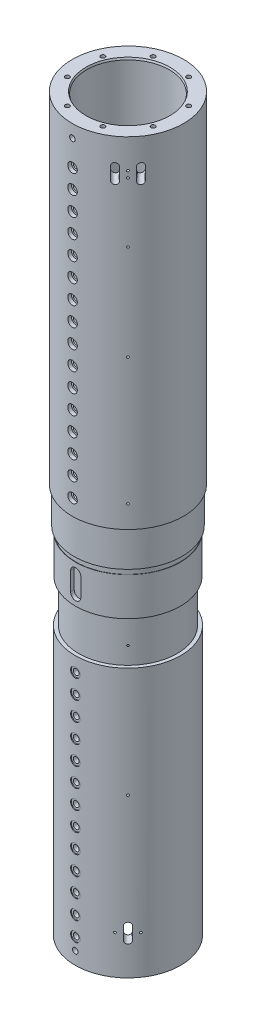
SolidWorks part; units mm, degrees
ref_plane "Front Plane" through (0, 0, 0) normal (0, 0, 1) x (1, 0, 0)
ref_plane "Top Plane" through (0, 0, 0) normal (0, 1, 0) x (1, 0, 0)
ref_plane "Right Plane" through (0, 0, 0) normal (1, 0, 0) x (0, 0, -1)
sketch "Sketch1" plane through (0, 0, 0) normal (0, 1, 0) x (1, 0, 0)
  circle A0 centre (0, 0) radius 65
  circle A1 centre (0, 0) radius 87.5
  dimension "D1" = 130
  dimension "D2" = 175
extrude "Boss-Extrude1" add sketch "Sketch1" along normal blind 1149
hole_wizard "M8 Tapped Hole1" positions "Sketch18" profile "Sketch19" tap size "M8" standard "GB"
sketch "Sketch18" plane through (0, 1149, 0) normal (0, 1, 0) x (1, 0, 0)
  line L0 (0, 0) -> (0, -111.092) construction
  line L2 (27.9359, -67.4432) -> (0, 0) construction
  circle A1 centre (0, 0) radius 73
  point P63 (27.9359, -67.4432)
  dimension "D1" = 146
  dimension "D2" = 22.5
sketch "Sketch19" plane through (27.9359, 1149, 67.4432) normal (1, 0, 0) x (0, 0, 1)
  line L0 (0, 0) -> (0, 33.2929)
  line L1 (0, 33.2929) -> (3.4, 31.25)
  line L2 (3.4, 31.25) -> (3.4, 0)
  line L5 (3.4, 0) -> (0, 0)
  line L10 (0, 33.2929) -> (-3.4, 31.25) construction
  line L11 (0, -6.35) -> (0, 107.95) construction
  dimension "螺纹孔钻头直径" = 6.8
  dimension "螺纹孔钻头深度" = 31.25
  dimension "导头角度" = 118
cosmetic thread "Cosmetic thread 5" parameters "D1"=25, "D2"=8
ref_plane "Plane1" through (0, 574.5, 0) normal (0, 1, 0) x (1, 0, 0)
hole_wizard "M8 Tapped Hole2" positions "Sketch20" profile "Sketch21" tap size "M8" standard "GB"
sketch "Sketch20" plane through (0, 0, 0) normal (0, -1, 0) x (-1, 0, 0)
  line L0 (0, 65) -> (0, 0) construction
  line L3 (0, 0) -> (-27.9359, -67.4432) construction
  circle A1 centre (0, 0) radius 65 construction
  point P0 (-27.9359, -67.4432)
  dimension "D1" = 22.5
  dimension "D2" = 73
sketch "Sketch21" plane through (27.9359, 0, 67.4432) normal (1, 0, 0) x (0, 0, -1)
  line L0 (0, 0) -> (0, 38.2929)
  line L1 (0, 38.2929) -> (3.4, 36.25)
  line L2 (3.4, 36.25) -> (3.4, 0)
  line L5 (3.4, 0) -> (0, 0)
  line L10 (0, 38.2929) -> (-3.4, 36.25) construction
  line L11 (0, -6.35) -> (0, 107.95) construction
  dimension "螺纹孔钻头直径" = 6.8
  dimension "螺纹孔钻头深度" = 36.25
  dimension "导头角度" = 118
cosmetic thread "Cosmetic thread 13" parameters "D1"=30, "D2"=8
pattern_circular "CirPattern1" count 8 over 360 about axis through (0, 0, 0) along (0, 1, 0) of "M8 Tapped Hole2"
ref_plane "Plane2" through (0, 0, 87.5) normal (0, 0, 1) x (1, 0, 0)
hole_wizard "Hole size (% based on socket head cap screw type)3" positions "Sketch23" profile "Sketch25" counterbore size "M8" standard "GB"
sketch "Sketch23" plane through (0, 0, 87.5) normal (0, 0, 1) x (1, 0, 0)
  line L0 (0, 1111.2839) -> (0, 0) construction
  line L3 (87.5, 1149) -> (-87.5, 1149) construction
  line L4 (-87.5, 0) -> (87.5, 0) construction
  point P0 (0, 1089)
  dimension "D1" = 60
sketch "Sketch25" plane through (0, 1089, 87.5) normal (1, 0, 0) x (0, -1, 0)
  line L0 (0, 0) -> (0, 82.7039)
  line L1 (0, 82.7039) -> (4.5, 80)
  line L2 (4.5, 80) -> (4.5, 6)
  line L3 (4.5, 6) -> (7.5, 6)
  line L4 (7.5, 6) -> (7.5, 0)
  line L5 (7.5, 0) -> (0, 0)
  line L10 (0, 82.7039) -> (-4.5, 80) construction
  line L11 (0, -6.35) -> (0, 107.95) construction
  dimension "孔直径" = 9
  dimension "孔深度" = 80
  dimension "柱形沉头孔直径" = 15
  dimension "柱形沉头孔深度" = 6
  dimension "导头角度" = 118
ref_plane "Plane3" through (61.8718, 0, 61.8718) normal (0.7071, 0, 0.7071) x (0, -1, 0)
sketch "Sketch29" plane through (61.8718, 0, 61.8718) normal (0.7071, 0, 0.7071) x (0, -1, 0)
  line L0 (-1108, 14.5) -> (-1088, 14.5) construction
  line L1 (-1108, 19.5) -> (-1088, 19.5)
  line L2 (-1108, 9.5) -> (-1088, 9.5)
  line L3 (-1108, -14.5) -> (-1088, -14.5) construction
  line L4 (-1108, -9.5) -> (-1088, -9.5)
  line L5 (-1108, -19.5) -> (-1088, -19.5)
  line L6 (-1149, 0) -> (-965.5167, 0) construction
  line L7 (-1149, 87.5) -> (-1149, -87.5) construction
  arc A0 (-1108, 19.5) -> (-1108, 9.5) centre (-1108, 14.5) ccw
  arc A1 (-1088, 9.5) -> (-1088, 19.5) centre (-1088, 14.5) ccw
  arc A2 (-1108, -9.5) -> (-1108, -19.5) centre (-1108, -14.5) ccw
  arc A3 (-1088, -19.5) -> (-1088, -9.5) centre (-1088, -14.5) ccw
  point P2 (-1098, 14.5)
  point P8 (-1098, -14.5)
  dimension "D1" = 29
  dimension "D2" = 5
  dimension "D3" = 41
  dimension "D4" = 20
extrude "Cut-Extrude13" cut sketch "Sketch29" against normal up to surface (25.494 mm away)
hole_wizard "M4 Tapped Hole2" positions "Sketch30" profile "Sketch31" tap size "M4" standard "GB"
sketch "Sketch30" plane through (61.8718, 0, 61.8718) normal (0.7071, 0, 0.7071) x (0, -1, 0)
  line L0 (-1098, 9.5) -> (-1098, -9.5) construction
  line L1 (-1108, 9.5) -> (-1088, 9.5) construction
  line L2 (-1088, -9.5) -> (-1108, -9.5) construction
  point P0 (-1103, 0)
  point P2 (-1093, 0)
  dimension "D1" = 10
sketch "Sketch31" plane through (61.8718, 1103, 61.8718) normal (0, 1, 0) x (0.7071, 0, -0.7071)
  line L0 (0, 0) -> (0, 12.4914)
  line L1 (0, 12.4914) -> (1.65, 11.5)
  line L2 (1.65, 11.5) -> (1.65, 0)
  line L5 (1.65, 0) -> (0, 0)
  line L10 (0, 12.4914) -> (-1.65, 11.5) construction
  line L11 (0, -6.35) -> (0, 107.95) construction
  dimension "螺纹孔钻头直径" = 3.3
  dimension "螺纹孔钻头深度" = 11.5
  dimension "导头角度" = 118
cosmetic thread "Cosmetic thread 18" parameters "D1"=8, "D2"=4
cosmetic thread "Cosmetic thread 19" parameters "D1"=8, "D2"=4
sketch "Sketch32" plane through (61.8718, 0, 61.8718) normal (0.7071, 0, 0.7071) x (0, -1, 0)
  line L0 (-51, 0) -> (-71, 0) construction
  line L1 (-51, -5) -> (-71, -5)
  line L2 (-51, 5) -> (-71, 5)
  line L4 (0, -87.5) -> (0, 87.5) construction
  arc A0 (-51, -5) -> (-51, 5) centre (-51, 0) ccw
  arc A1 (-71, 5) -> (-71, -5) centre (-71, 0) ccw
  point P2 (-61, 0)
  dimension "D1" = 5
  dimension "D3" = 51
  dimension "D2" = 20
extrude "Cut-Extrude14" cut sketch "Sketch32" against normal up to surface (22.6926 mm away)
hole_wizard "M4 Tapped Hole3" positions "Sketch33" profile "Sketch34" tap size "M4" standard "GB"
sketch "Sketch33" plane through (61.8718, 0, 61.8718) normal (0.7071, 0, 0.7071) x (0, -1, 0)
  line L0 (-46, 0) -> (-76, 0) construction
  line L3 (-61, 5) -> (-61, 12.6978) construction
  line L4 (-71, 5) -> (-51, 5) construction
  arc A0 (-51, -5) -> (-51, 5) centre (-51, 0) ccw construction
  arc A1 (-71, 5) -> (-71, -5) centre (-71, 0) ccw construction
  point P0 (-61, 14.5)
  point P2 (-61, -14.5)
  dimension "D1" = 29
sketch "Sketch34" plane through (72.1249, 61, 51.6188) normal (0, 1, 0) x (0.7071, 0, -0.7071)
  line L0 (0, 0) -> (0, 12.4914)
  line L1 (0, 12.4914) -> (1.65, 11.5)
  line L2 (1.65, 11.5) -> (1.65, 0)
  line L5 (1.65, 0) -> (0, 0)
  line L10 (0, 12.4914) -> (-1.65, 11.5) construction
  line L11 (0, -6.35) -> (0, 107.95) construction
  dimension "螺纹孔钻头直径" = 3.3
  dimension "螺纹孔钻头深度" = 11.5
  dimension "导头角度" = 118
cosmetic thread "Cosmetic thread 20" parameters "D1"=8, "D2"=4
cosmetic thread "Cosmetic thread 21" parameters "D1"=8, "D2"=4
hole_wizard "G1/8 Tapped Hole1" positions "Sketch43" profile "Sketch44" tap size "G1/8" standard "GB"
sketch "Sketch43" plane through (0, 0, 87.5) normal (0, 0, 1) x (1, 0, 0)
  line L0 (0, 0) -> (0, 20) construction
  line L1 (87.5, 1149) -> (-87.5, 1149) construction
  point P0 (0, 20)
  point P7 (0, 1129)
  dimension "D1" = 20
  dimension "D2" = 20
sketch "Sketch44" plane through (0, 20, 87.5) normal (1, 0, 0) x (0, -1, 0)
  line L0 (0, 0) -> (0, 24.8238)
  line L1 (0, 24.8238) -> (4.4, 22.18)
  line L2 (4.4, 22.18) -> (4.4, 0)
  line L5 (4.4, 0) -> (0, 0)
  line L10 (0, 24.8238) -> (-4.4, 22.18) construction
  line L11 (0, -6.35) -> (0, 107.95) construction
  dimension "螺纹孔钻头直径" = 8.8
  dimension "螺纹孔钻头深度" = 22.18
  dimension "导头角度" = 118
cosmetic thread "Cosmetic thread 44" parameters "D1"=19.46, "D2"=9.728
cosmetic thread "Cosmetic thread 48" parameters "D1"=19.46, "D2"=9.728
hole_wizard "M4 Tapped Hole4" positions "Sketch45" profile "Sketch46" tap size "M4" standard "GB"
sketch "Sketch45" plane through (61.8718, 0, 61.8718) normal (0.7071, 0, 0.7071) x (0, -1, 0)
  line L0 (-1093, 0) -> (-999, 0)
  line L1 (-1149, 87.5) -> (-1149, -87.5) construction
  point P0 (-999, 0)
  point P2 (-849, 0)
  point P13 (-649, 0)
  point P15 (-449, 0)
  point P17 (-249, 0)
  dimension "D1" = 150
  dimension "D2" = 150
  dimension "D3" = 200
  dimension "D4" = 200
  dimension "D5" = 200
sketch "Sketch46" plane through (61.8718, 999, 61.8718) normal (0, 1, 0) x (0.7071, 0, -0.7071)
  line L0 (0, 0) -> (0, 12.4914)
  line L1 (0, 12.4914) -> (1.65, 11.5)
  line L2 (1.65, 11.5) -> (1.65, 0)
  line L5 (1.65, 0) -> (0, 0)
  line L10 (0, 12.4914) -> (-1.65, 11.5) construction
  line L11 (0, -6.35) -> (0, 107.95) construction
  dimension "螺纹孔钻头直径" = 3.3
  dimension "螺纹孔钻头深度" = 11.5
  dimension "导头角度" = 118
cosmetic thread "Cosmetic thread 25" parameters "D1"=0, "D2"=4.3
cosmetic thread "Cosmetic thread 26" parameters "D1"=0, "D2"=4.3
cosmetic thread "Cosmetic thread 27" parameters "D1"=0, "D2"=4.3
cosmetic thread "Cosmetic thread 28" parameters "D1"=0, "D2"=4.3
cosmetic thread "Cosmetic thread 29" parameters "D1"=0, "D2"=4.3
sketch "Sketch47" plane through (0, 0, 0) normal (0, 1, 0) x (1, 0, 0)
  circle A0 centre (0, 0) radius 85
  circle A1 centre (0, 0) radius 141.9465
  dimension "D1" = 170
extrude "Cut-Extrude19" cut sketch "Sketch47" along normal blind 614
sketch "Sketch48" plane through (0, 614, 0) normal (0, -1, 0) x (1, 0, 0)
  circle A0 centre (0, 0) radius 82
  circle A1 centre (0, 0) radius 100.4458
  dimension "D1" = 164
extrude "Cut-Extrude20" cut sketch "Sketch48" along normal blind 9 from offset 56
sketch "Sketch54" plane through (0, 0, 0) normal (0, -1, 0) x (1, 0, 0)
  circle A0 centre (0, 0) radius 83
  dimension "D1" = 166
extrude "Cut-Extrude26" cut sketch "Sketch54" against normal blind 550 flip side to cut
sketch "Sketch55" plane through (0, 558, 0) normal (0, -1, 0) x (1, 0, 0)
  circle A0 centre (0, 0) radius 82.5
  dimension "D1" = 165
extrude "Cut-Extrude27" cut sketch "Sketch55" along normal blind 69 flip side to cut
sketch "Sketch56" plane through (0, 489, 0) normal (0, 1, 0) x (1, 0, 0)
  circle A0 centre (0, 0) radius 77.5
  dimension "D1" = 155
extrude "Cut-Extrude28" cut sketch "Sketch56" against normal blind 67 flip side to cut
sketch "Sketch57" plane through (0, 0, 0) normal (0, -1, 0) x (1, 0, 0)
  circle A0 centre (0, 0) radius 67.5
  dimension "D1" = 135
extrude "Cut-Extrude29" cut sketch "Sketch57" against normal blind 14
sketch "Sketch58" plane through (0, 0, 87.5) normal (0, 0, 1) x (1, 0, 0)
  line L0 (0, 504.5) -> (0, 533.5) construction
  line L1 (-8, 504.5) -> (-8, 533.5)
  line L2 (8, 504.5) -> (8, 533.5)
  line L3 (-82.5, 489) -> (82.5, 489) construction
  arc A0 (-8, 504.5) -> (8, 504.5) centre (0, 504.5) ccw
  arc A1 (8, 533.5) -> (-8, 533.5) centre (0, 533.5) ccw
  point P3 (0, 519)
  dimension "D1" = 8
  dimension "D2" = 29
  dimension "D3" = 30
extrude "Cut-Extrude30" cut sketch "Sketch58" against normal blind 11
pattern_circular "CirPattern2" count 8 over 360 about axis through (0, 0, 0) along (0, 1, 0) of "M8 Tapped Hole1"
pattern_linear "LPattern1" count 36 spacing 30 along (0, -1, 0) skipping (16, 0), (17, 0), (18, 0), (19, 0), (20, 0), (21, 0), (22, 0) of "Hole size (% based on socket head cap screw type)3"
chamfer "Chamfer1" distance 3 angle 20 2 edges at (0, 1149, 65) (0, 0, -67.5)
chamfer "Chamfer2" distance 2 angle 20 1 edges at (0, 14, -65)
